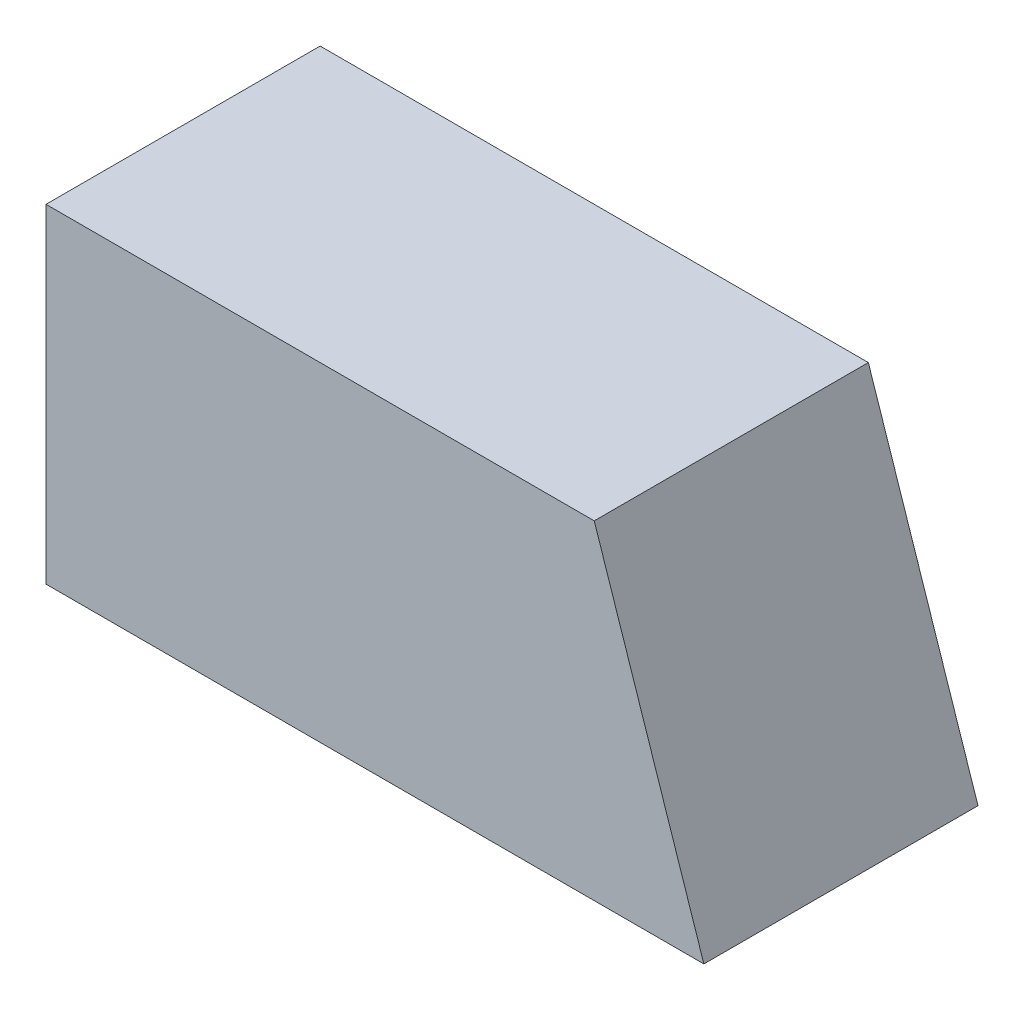
from build123d import *

# Parameters (mm, degrees)
BOSS_EXTRUDE1_DEPTH = 500


with BuildPart() as part:
    # Sketch1 → Boss-Extrude1 (new body)
    with BuildSketch(Plane.XY):
        Polygon((0, 0), (0, 600), (1000, 600), (1200, 0), align=None)
    extrude(amount=BOSS_EXTRUDE1_DEPTH)


solid = part.part
